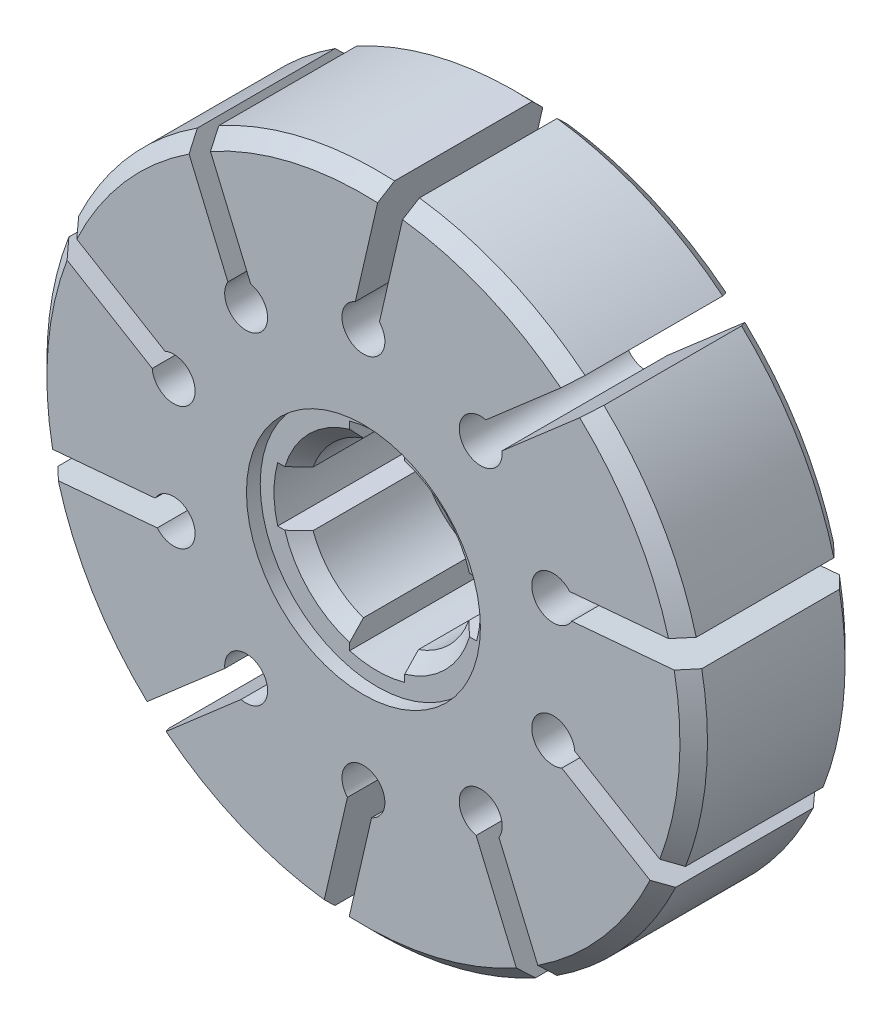
SolidWorks part; units mm, degrees
ref_plane "前视基准面" through (0, 0, 0) normal (0, 0, 1) x (1, 0, 0)
ref_plane "上视基准面" through (0, 0, 0) normal (0, 1, 0) x (1, 0, 0)
ref_plane "右视基准面" through (0, 0, 0) normal (1, 0, 0) x (0, 0, -1)
sketch "草图1" plane through (0, 0, 0) normal (0, 0, 1) x (1, 0, 0)
  circle A0 centre (0, 0) radius 24
extrude "凸台-拉伸1" add sketch "草图1" along normal blind 12
chamfer "倒角1" distance 1 angle 45 2 edges at (24, 0, 0) (24, 0, 12)
sketch "草图2" plane through (0, 0, 12) normal (0, 0, 1) x (1, 0, 0)
  circle A0 centre (0, 0) radius 8.5
extrude "切除-拉伸1" cut sketch "草图2" against normal blind 1
sketch "草图3" plane through (0, 0, 0) normal (0, 0, -1) x (-1, 0, 0)
  circle A0 centre (0, 0) radius 8.5
extrude "切除-拉伸2" cut sketch "草图3" against normal blind 1
sketch "草图4" plane through (0, 0, 11) normal (0, 0, 1) x (1, 0, 0)
  circle A0 centre (0, 0) radius 6
extrude "切除-拉伸3" cut sketch "草图4" against normal through all
chamfer "倒角2" distance 1 angle 45 2 edges at (-6, 0, 1) (6, 0, 11)
sketch "草图5" plane through (0, 0, 11) normal (0, 0, 1) x (1, 0, 0)
  line L0 (-10.1907, 0) -> (2, 0) construction
  line L1 (0, 10.279) -> (0, 0) construction
  line L2 (-2, 7.2284) -> (-2, 2)
  line L3 (2, 7.2284) -> (2, 2)
  line L4 (-7.2284, 2) -> (-2, 2)
  line L5 (-7.2284, -2) -> (-2, -2)
  line L6 (2, 2) -> (7.2284, 2)
  line L7 (-2, -2) -> (-2, -5.6569)
  line L8 (0, -2) -> (0, -11.0923) construction
  line L9 (2, -2) -> (2, -5.6569)
  line L10 (7.5, 0) -> (13.5604, 0) construction
  line L11 (-2, -5.6569) -> (-2, -7.2284)
  line L12 (2, -5.6569) -> (2, -7.2284)
  line L13 (2, -2) -> (7.2284, -2)
  arc A0 (-7.2284, 2) -> (-7.2284, -2) centre (0, 0) ccw
  circle A1 centre (0, 0) radius 6 construction
  arc A2 (2, 7.2284) -> (-2, 7.2284) centre (0, 0) ccw
  arc A3 (-2, -7.2284) -> (2, -7.2284) centre (0, 0) ccw
  arc A4 (7.2284, -2) -> (7.2284, 2) centre (0, 0) ccw
  dimension "D1" = 2
  dimension "D2" = 2
  dimension "D3" = 2
  dimension "D4" = 2
extrude "切除-拉伸4" cut sketch "草图5" against normal through all
sketch "草图6" plane through (0, 0, 12) normal (0, 0, 1) x (1, 0, 0)
  line L0 (0, 15.574) -> (0, 0) construction
  line L1 (0, 14.5) -> (2.7428, 26.3802) construction
  line L2 (0, 14.5) -> (0, 0) construction
  line L4 (1.1635, 15.5388) -> (3.3536, 25.025)
  line L5 (-0.5904, 15.9437) -> (1.5644, 25.277)
  line L6 (1.5644, 25.277) -> (3.3536, 25.025)
  arc A0 (-0.5904, 15.9437) -> (1.1635, 15.5388) centre (0, 14.5) ccw
  dimension "D3" = 0.9
  dimension "D1" = 14.5
  dimension "D2" = 13
  dimension "D4" = 0.9
extrude "切除-拉伸5" cut sketch "草图6" against normal through all
pattern_circular "阵列(圆周)1" count 10 over 360 about axis through (0, 0, 0) along (0, 0, 1) of "切除-拉伸5"
